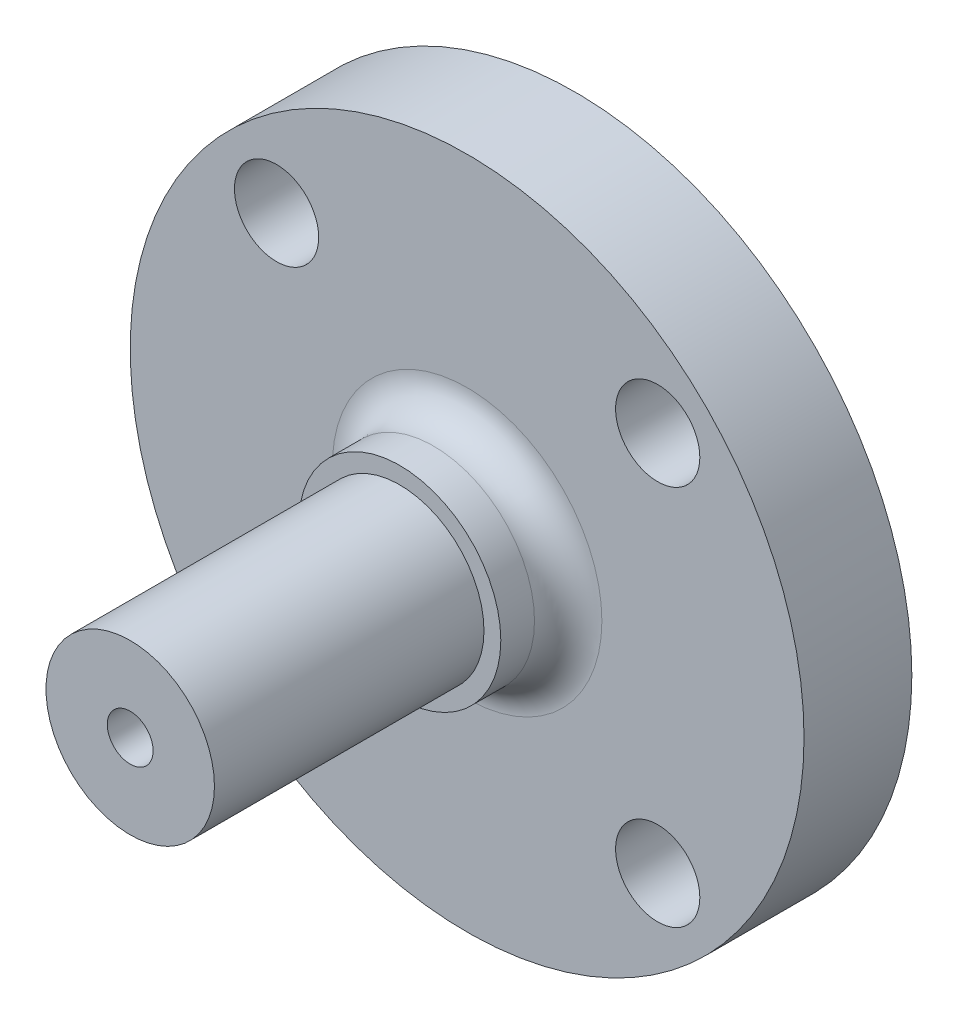
SolidWorks part; units mm, degrees
ref_plane "前视基准面" through (0, 0, 0) normal (0, 0, 1) x (1, 0, 0)
ref_plane "上视基准面" through (0, 0, 0) normal (0, 1, 0) x (1, 0, 0)
ref_plane "右视基准面" through (0, 0, 0) normal (1, 0, 0) x (0, 0, -1)
sketch "草图1" plane through (0, 0, 0) normal (0, 0, 1) x (1, 0, 0)
  circle A0 centre (0, 0) radius 50
  dimension "D1" = 100
extrude "凸台-拉伸1" add sketch "草图1" along normal blind 16
sketch "草图2" plane through (0, 0, 16) normal (0, 0, 1) x (1, 0, 0)
  circle A0 centre (0, 0) radius 15
  dimension "D1" = 30
extrude "凸台-拉伸2" add sketch "草图2" along normal blind 10
sketch "草图3" plane through (0, 0, 26) normal (0, 0, 1) x (1, 0, 0)
  circle A0 centre (0, 0) radius 12.5
  dimension "D1" = 25
extrude "凸台-拉伸3" add sketch "草图3" along normal blind 40
hole_wizard "Ø12.5 (12.5) 直径孔1" positions "草图4" profile "草图5" hole size "Ø12.5" standard "GB" end condition through all
sketch "草图4" plane through (0, 0, 16) normal (0, 0, 1) x (1, 0, 0)
  line L0 (-28.2843, 28.2843) -> (0, 0) construction
  line L1 (0, 0) -> (0, 57.1924) construction
  point P0 (-28.2843, 28.2843)
  dimension "D1" = 45
  dimension "D2" = 40
sketch "草图5" plane through (-28.2843, 28.2843, 16) normal (1, 0, 0) x (0, -1, 0)
  line L0 (0, 0) -> (0, 16)
  line L1 (0, 16) -> (6.25, 16)
  line L2 (6.25, 16) -> (6.25, 0)
  line L5 (6.25, 0) -> (0, 0)
  line L11 (0, -6.35) -> (0, 107.95) construction
  dimension "通孔孔直径" = 12.5
  dimension "通孔孔深度" = 16
pattern_circular "阵列(圆周)1" count 4 over 360 about axis through (0, 0, 0) along (0, 0, 1) of "Ø12.5 (12.5) 直径孔1"
hole_wizard "M8 螺纹孔1" positions "草图6" profile "草图7" tap size "M8" standard "GB"
sketch "草图6" plane through (0, 0, 66) normal (0, 0, 1) x (1, 0, 0)
  point P0 (0, 0)
sketch "草图7" plane through (0, 0, 66) normal (1, 0, 0) x (0, -1, 0)
  line L0 (0, 0) -> (0, 21.7929)
  line L1 (0, 21.7929) -> (3.4, 19.75)
  line L2 (3.4, 19.75) -> (3.4, 0)
  line L5 (3.4, 0) -> (0, 0)
  line L10 (0, 21.7929) -> (-3.4, 19.75) construction
  line L11 (0, -6.35) -> (0, 107.95) construction
  dimension "螺纹孔钻头直径" = 6.8
  dimension "螺纹孔钻头深度" = 19.75
  dimension "导头角度" = 118
cosmetic thread "孔螺蚊线1" parameters "D1"=16, "D2"=8
fillet "圆角1" radius 5 1 edges at (15, 0, 16)
